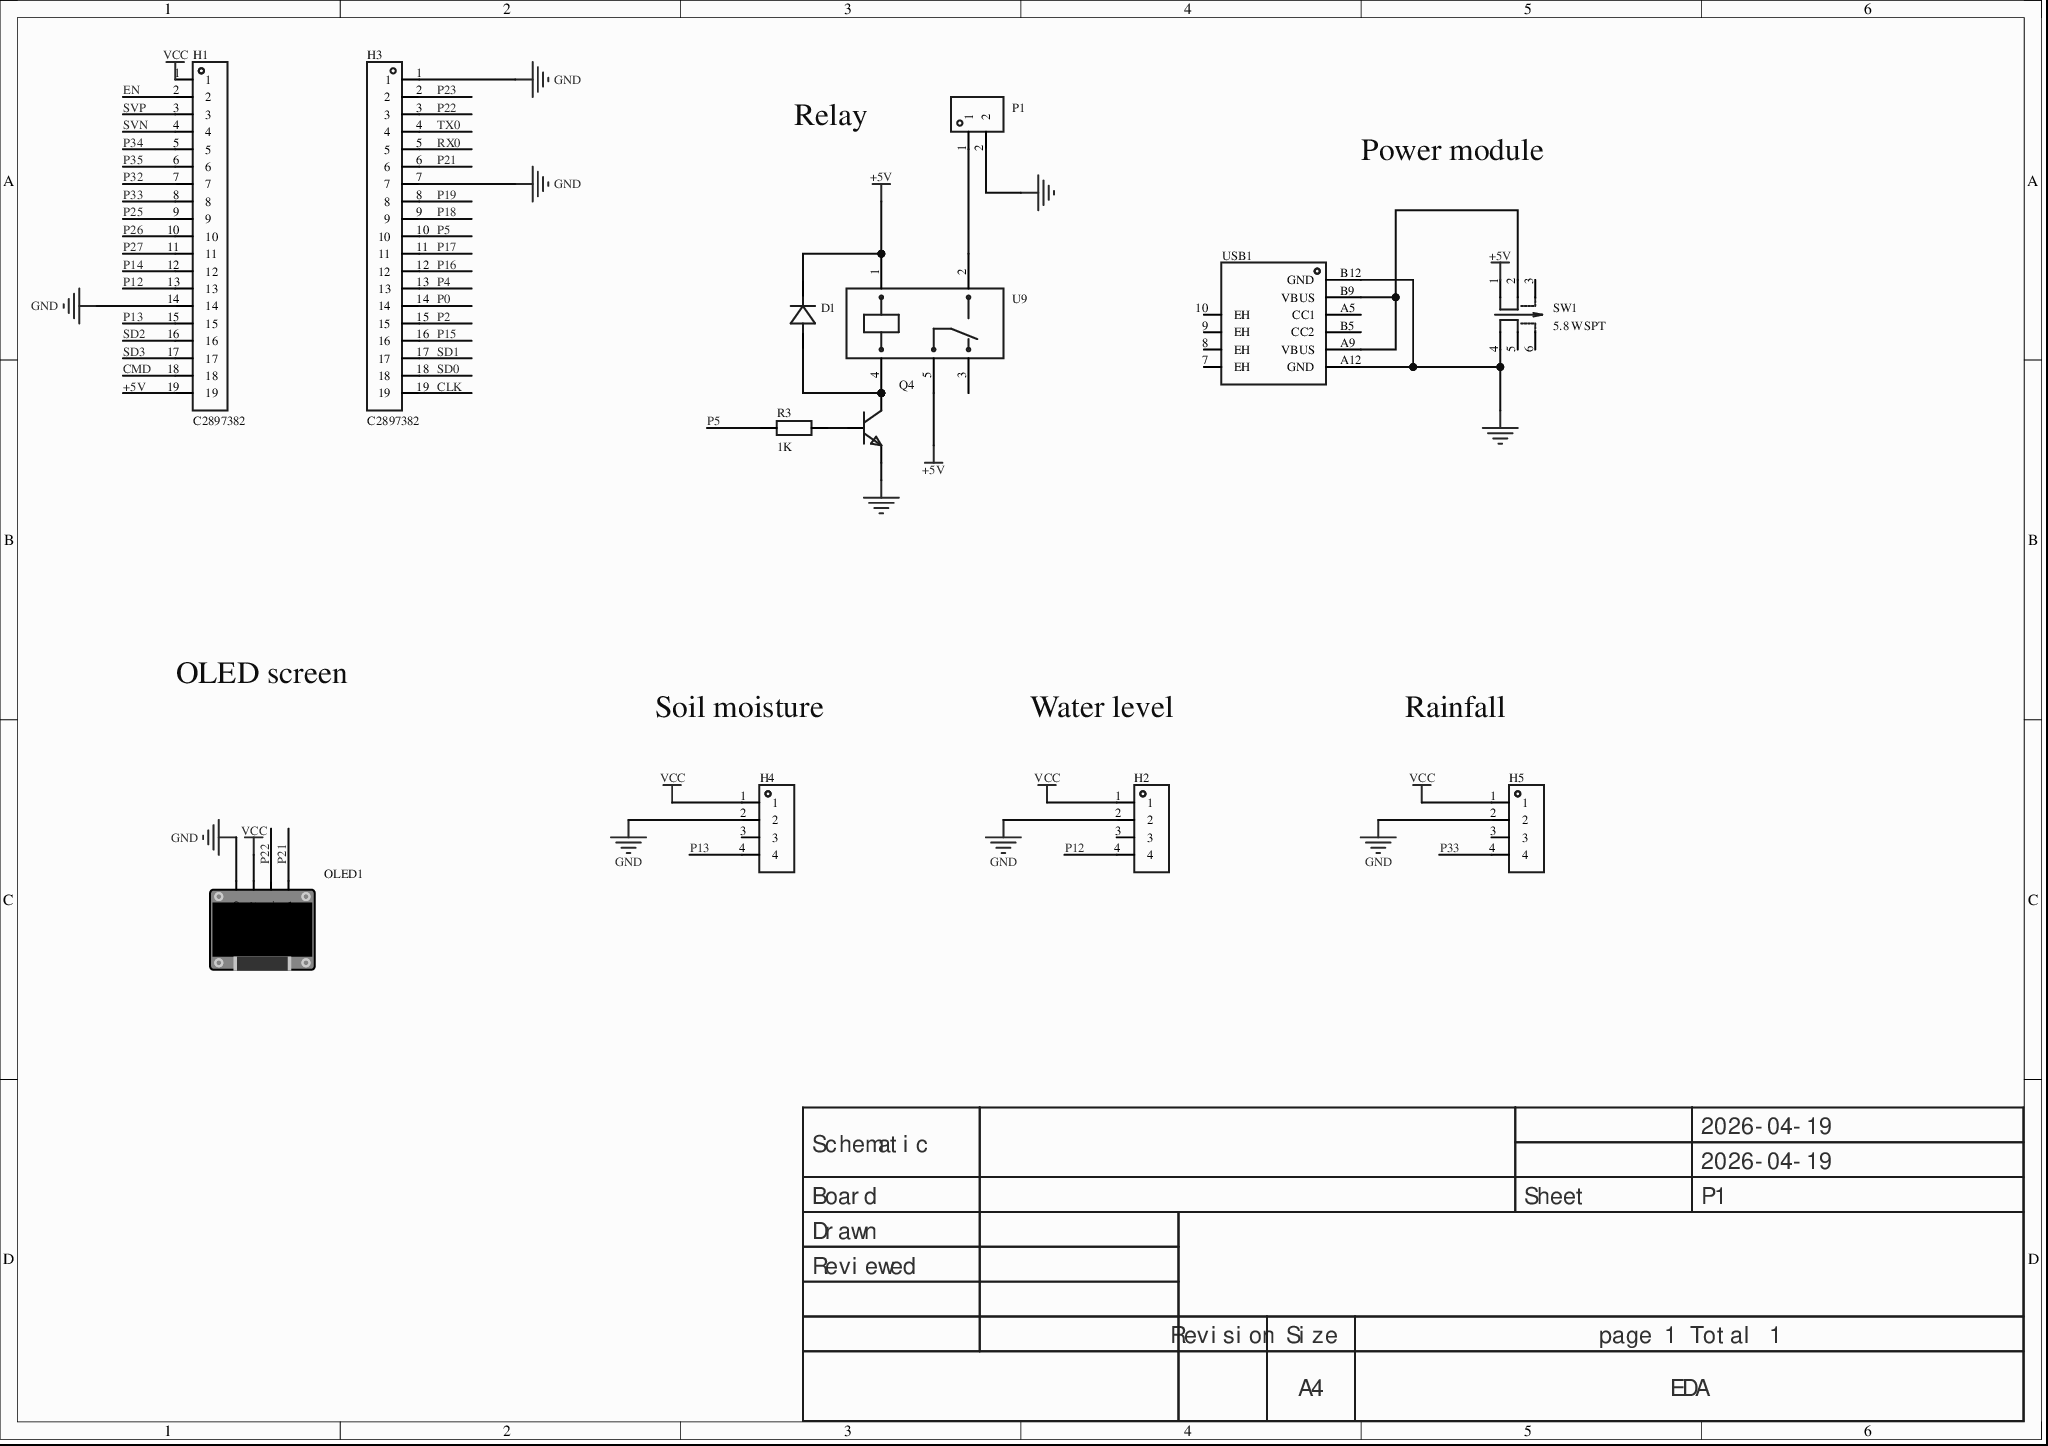
[diagram p0: MISC89058-3.schdoc]
# Altium project MISC89058-2.PrjPcb
1 sheet, 13 parts. Net scope: global (net labels, ports and power ports of the same name join across sheets).
Board file: MISC89058.pcbdoc

## Sheet MISC89058-3.schdoc
size 297 x 209 mm; Version: V1.0; @Project Name: MISC89058; @Page Count: 1; @Update Date: 2026-04-19; @Create Date: 2026-04-19; @Schematic Name: MISC89058; @Page No: 1; @Create Time: 19:02:24; @Update Time: 19:02:29; @Board Name: MISC89058

### Parts
D1  (no value)  [DO_1N4007]
H1  C2897382  [HDR-TH_19P-P2.54-V-F]
H2  (no value)  [HDR-TH_4P-P2.54-V-F]
H3  C2897382  [HDR-TH_19P-P2.54-V-F]
H4  (no value)  [HDR-TH_4P-P2.54-V-F]
H5  (no value)  [HDR-TH_4P-P2.54-V-F]
OLED1  (no value)  [0.96OLED_4P]
P1  WAFER-XH254Z-2A  [CONN-TH_2P-P2.50_XH-2A_3045048]  (value not drawn)
Q4  (no value)  [S8050_TO_92]
R3  1K  [Res_1/8W]
SW1  5.8 WSPT  [SW-TH_6P-L5.8-W5.8-P2.00-LS4.5-TL_K8-5851E-L1]
U9  SRD-12VDC-SL-C  [RELAY-TH_SRD-XXVDC-XL-C]  (value not drawn)
USB1  (no value)  [USB_ TYPE-C-6P]

### Nets
+5V: D1.1(K) H1.19 SW1.1 U9.1 U9.5
GND: H1.14 H2.2 H3.1 H3.7 H4.2 H5.2 OLED1.1(GND) P1.2 Q4.1(E) SW1.4 USB1.A12(GND) USB1.B12(GND)
VCC: H1.1 H2.1 H4.1 H5.1 OLED1.2(VCC)
CLK: H3.19
CMD: H1.18
EN: H1.2
P0: H3.14
P2: H3.15
P4: H3.13
P5: H3.10 R3.1
P12: H1.13 H2.4
P13: H1.15 H4.4
P14: H1.12
P15: H3.16
P16: H3.12
P17: H3.11
P18: H3.9
P19: H3.8
P21: H3.6 OLED1.4(SDA)
P22: H3.3 OLED1.3(SCL)
P23: H3.2
P25: H1.9
P26: H1.10
P27: H1.11
P32: H1.7
P33: H1.8 H5.4
P34: H1.5
P35: H1.6
RX0: H3.5
SD0: H3.18
SD1: H3.17
SD2: H1.16
SD3: H1.17
SVN: H1.4
SVP: H1.3
TX0: H3.4
NetD1_2: D1.2(A) Q4.3(C) U9.4
NetP1_1: P1.1 U9.2
NetQ4_2: Q4.2(B) R3.2
NetSW1_2: SW1.2 USB1.A9(VBUS) USB1.B9(VBUS)

Not connected (* = marked no-connect by the designer): H2 3; H4 3; H5 3; SW1 3 5 6; U9 3; USB1 7(EH) 8(EH) 9(EH) 10(EH) A5(CC1) B5(CC2)

### Notes on the sheet
- Relay
- Power module
- OLED screen
- Soil moisture
- Water level
- Rainfall
- 2026-04-19
- Schematic
- Board
- Sheet
- P1
- Drawn
- Reviewed
- Revision
- Size
- A4
- page 1 Total 1
- EDA

### Library data of the parts
D1 = D_1N4007A: AddInBom: yes; ModelId: 6de1e9b71a0d4751b4e9df530304c1a3; ModelName: DO-41_D2.4-L4.7-P8.70; ModelTransform: 373.9,94.4,232.29,0,0,0,0,0,-140; Symbol: D_1N4007; Device: D_1N4007A; Supplier Footprint: DO-41; ConvertToPcb: yes; FootprintName: DO_1N4007
H1 H3 = HDR-F_2.54_1x19P: ConvertToPcb: yes; ModelId: 131ee080550a465daf9368d356f53fe90819f05c4eef4c71ace90d822a990e87; ModelName: HDR-TH_19P-P2.54-F-LI-1X19P; ModelTransform: 1919.68128,95.6691,0,0,0,0,0,0,-125.984; Symbol: HDR-F_2.54_1x19P; Device: HDR-F_2.54_1x19P; AddInBom: yes; Supplier Footprint: 插件; ManufacturerPart: C2897382; FootprintName: HDR-TH_19P-P2.54-V-F
H2 H4 H5 = HDR-F_2.54_1x4P: Symbol: 2.54-1*4P female; 3D Model: d187812051054f85879fcaa51a310d8e0819f05c4eef4c71ace90d822a990e87; 3D Model Transform: 419.6842,98.464,0,0,0,0,0,0,-118.11; ConvertToPcb: yes; Device: HDR-F_2.54_1x4P; Supplier Part: C2718488; Supplier Footprint: 插件; FootprintName: HDR-TH_4P-P2.54-V-F; AddInBom: yes; ModelName: HDR-TH_4P-P2.54-V-F
OLED1 = 0.96OLED模块_4P: Symbol: 0.96OLED module_4P; ConvertToPcb: yes; ModelId: 79c000fdb68d45a296c2e9bedf4f90550819f05c4eef4c71ace90d822a990e87; ModelTransform: 1393.69792,1318.895,0,0,0,0,0,-560.079,-137.795; Device: 0.96OLED module_4P; AddInBom: yes; FootprintName: 0.96OLED_4P; Supplier Footprint: 插件; ModelName: 0.96OLED_4P
P1 = WAFER-XH254Z-2A: Pin structure: 1x2P; Pitch: 2.54mm; Mounting: through-hole; Reference series: XH; Total pins: 2P; Rows: 1; Pins per row: 2; Rated current: 3A; Operating temperature range: -25℃~+85℃;; Manufacturer: HANBO(汉博); AddInBom: yes; ModelId: a03ee9acfa8e4e25b912a99a3551fb92; ModelTransform: 295.275,228.7397,0,0,0,0,0,21.654,-133.858; Number of PINs Per Row: 2; Symbol: WAFER-XH254Z-2A; Device: WAFER-XH254Z-2A; LCSC Part Name: WAFER-XH254Z-2A; SupplierPart: C7432682; ManufacturerPart: WAFER-XH254Z-2A; Supplier Footprint: 插件,P=2.5mm; JLCPCB Part Class: Extended library; Datasheet: https://atta.szlcsc.com/upload/public/pdf/source/20230718/3B4FABA5D38EFB02DAF74E7C2B33D98F.pdf; Supplier: LCSC; ConvertToPcb: yes; FootprintName: CONN-TH_2P-P2.50_XH-2A_3045048; ModelName: CONN-TH_2P-P2.50_XH-2A_3045048; Pins Structure: 1x2P; Mounting Style: Through-hole; Reference Series: XH; Number of Pins: 2P; Number of Rows: 1; Current Rating (Max): 3A; Operating Temperature Range: -25℃~+85℃
Q4 = S8050_TO_NPN: ConvertToPcb: yes; ModelId: aafe8e06f2154e7c93506efd0d6632dd; ModelName: TO-92-3_L4.9-W3.7-P1.27-L; ModelTransform: 180.78,141.44,417.3,0,0,0,0,0,-200; Device: S8050_TO_NPN; Symbol: S8050_TO_NPN; AddInBom: yes; Supplier Footprint: TO-92; FootprintName: S8050_TO_92
R3 = Res_AXIAL-1/8W: Symbol: Resistor; ConvertToPcb: yes; Value: 10kΩ; ModelId: b2b5ae7ae4c642178fe0039925c86a3f; ModelName: RES-TH_BD1.8-L3.2-P7.20-D0.4; ModelTransform: 282.86,66.88,253.09,0,0,0,0,0,-191; Device: Res_AXIAL-1/8W; AddInBom: yes; Supplier Footprint: 轴向引线; FootprintName: Res_1/8W
SW1 = 5.8 WSPT: Circuit structure: DPDT; Self-lock/no-lock: no lock; Mounting: through-hole; Contact current: 100mA; Rated voltage (AC): -; Rated voltage (DC): 30V; With lamp: no; Actuating force: 1.8N; Mechanical life: 5 thousand cycles;; Manufacturer: SHOU HAN(首韩); AddInBom: yes; ModelId: b8faad98a5c645e9866333cdaba903c3; ModelTransform: 229.1334,228.346,0,0,0,0,0,0,-137.795; Self Lock / No Lock: No lock; Actuator Style: Rectangular plunger; Insulation Resistance: 100MΩ; Actuator/Cap Color: Blue; With Lamp: Without lamp; Pin Style: PC pin; Symbol: 5.8 WSPT; Device: 5.8 WSPT; LCSC Part Name: 按键开关5.8x5.8 无锁平头 180gf; SupplierPart: C5379898; ManufacturerPart: 5.8 WSPT; Supplier Footprint: 插件; JLCPCB Part Class: Extended library; Datasheet: https://atta.szlcsc.com/upload/public/pdf/source/20230323/C831DDA43A625CDC196CB35781CDAE7F.pdf; Supplier: LCSC; ConvertToPcb: yes; FootprintName: SW-TH_6P-L5.8-W5.8-P2.00-LS4.5-TL_K8-5851E-L1; ModelName: SW-TH_6P-L5.8-W5.8-P2.00-LS4.5-TL_K8-5851E-L1; Circuit: DPDT; IP Rating: -; Mounting Style: Through-hole; Contact Current: 100mA; Voltage Rating (AC): -; Voltage Rating (DC): 30V; Operating Force: 1.8N; Operating Temperature: -10℃~+70℃; Mechanical Life: 5 thousand cycles
U9 = SRD-12VDC-SL-C: Coil voltage: 12V; Contact form: one changeover group: 1C (SPDT); Contact rating (resistive load): -; Max switching voltage: 250V@AC; Max switching current: 15A;; Manufacturer: 松乐; AddInBom: yes; ModelId: d0eda9b8bf8746d18ae810ab88dc78e7; ModelName: RELAY-TH_L19.2-W15.6-H15.8; ModelTransform: 755.904,622.4397,0,0,0,0,34.882,0,-118.11; Pin Number: 5; Coil Rated Power: 360mW; Coil Type: Non-polar, single coil; Coil Resistance: 400Ω; Contact Resistance: 100mΩ; Operate Time: 10ms; Symbol: SRD-12VDC-SL-C; Device: SRD-12VDC-SL-C; LCSC Part Name: SRD-12VDC-SL-C; SupplierPart: C30431; ManufacturerPart: SRD-12VDC-SL-C; Supplier Footprint: 插件,15.6x19.2mm; JLCPCB Part Class: Extended library; Datasheet: https://atta.szlcsc.com/upload/public/pdf/source/20200305/C490149_C96E4098A3B1FFB377D5AD2E40B7C2A8.pdf; Supplier: LCSC; ConvertToPcb: yes; FootprintName: RELAY-TH_SRD-XXVDC-XL-C; Coil Voltage: 12V; Contact Form: One changeover group: 1C (SPDT); Contact Rating: -; Maximum Switching Voltage: 250V@AC; Maximum Switching Current: 15A; Release Time: 10ms
USB1 = USB_ Type-C-6P: AddInBom: yes; ModelId: d4f492a4e6024845a13b3f6a4ef2d2cb0819f05c4eef4c71ace90d822a990e87; ModelName: USB-SMD_U262-061N-4BVC11; ModelTransform: 352.362,281.496,0,0,0,0,0,-47.244,-39.37; Symbol: USB_ TYPE-C-6P; Device: USB_ Type-C-6P; Supplier Footprint: SMD; ConvertToPcb: yes; FootprintName: USB_ TYPE-C-6P